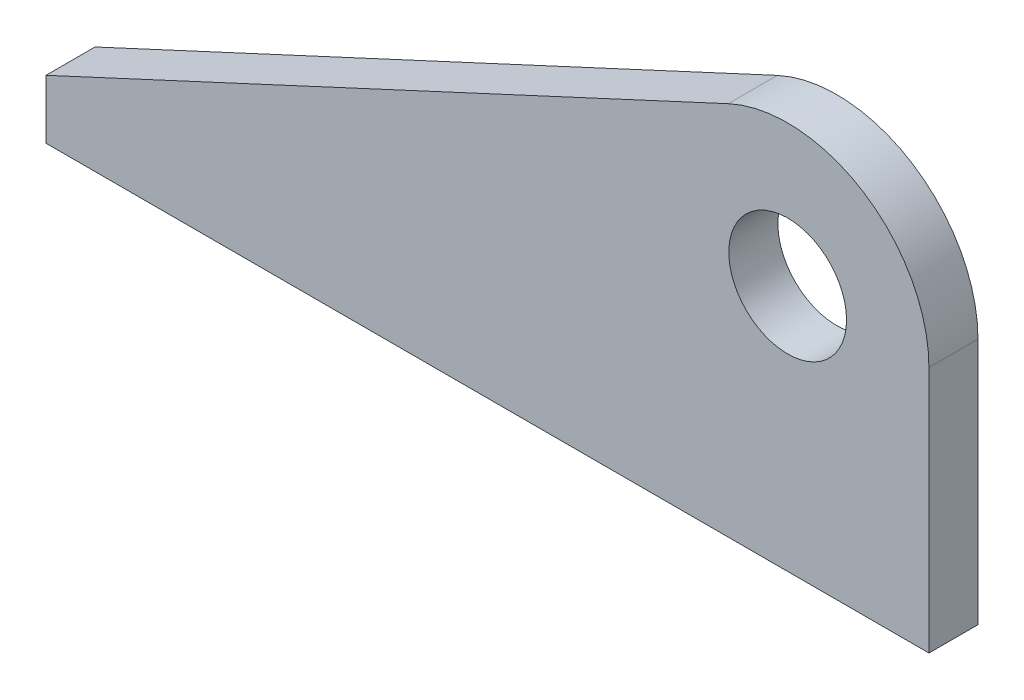
from build123d import *

# Parameters (mm, degrees)
SKETCH1_R           = 30
BOSS_EXTRUDE1_DEPTH = 25


with BuildPart() as part:
    # Sketch1 → Boss-Extrude1 (new body)
    with BuildSketch(Plane.XY):
        with BuildLine():
            Line((0, 0), (0, 30))
            Line((0, 30), (347.698254159, 191.313124248))
            ThreePointArc((347.698254159, 191.313124248), (416.744511221, 186.68659531), (450, 126))
            Line((450, 126), (450, 0))
            Line((450, 0), (0, 0))
        make_face()
        with Locations((378, 126)):
            Circle(SKETCH1_R, mode=Mode.SUBTRACT)
    extrude(amount=BOSS_EXTRUDE1_DEPTH)


solid = part.part
